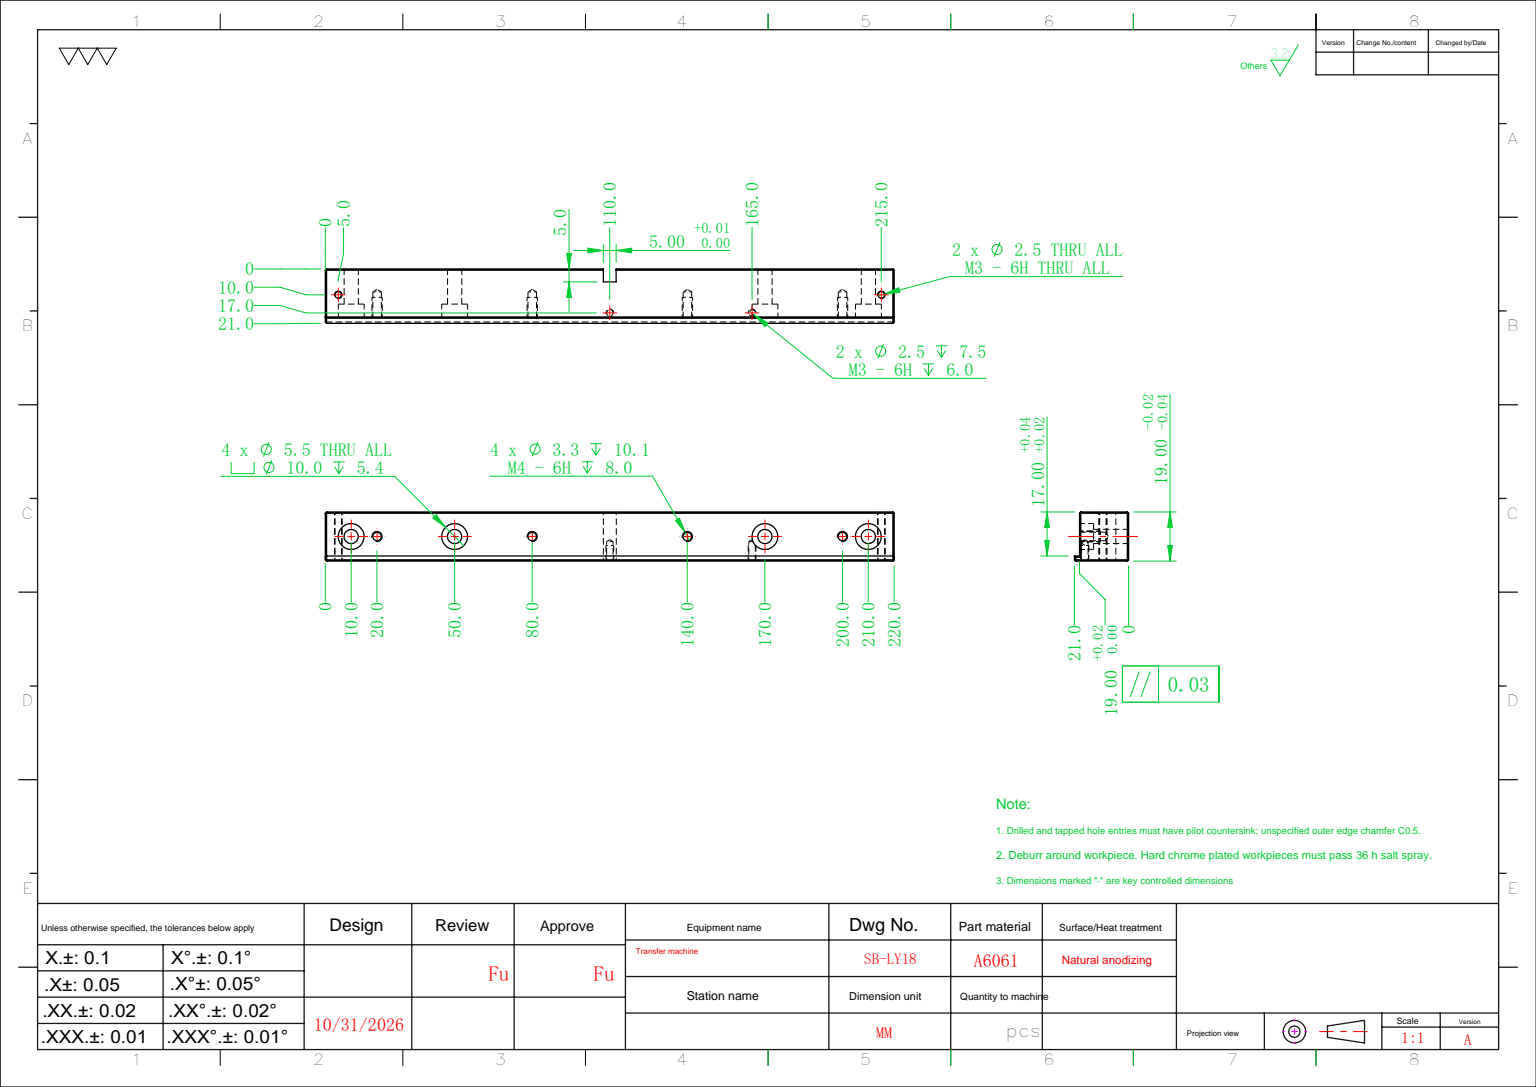
SolidWorks part; units mm, degrees
ref_plane "前视基准面" through (0, 0, 0) normal (0, 0, 1) x (1, 0, 0)
ref_plane "上视基准面" through (0, 0, 0) normal (0, 1, 0) x (1, 0, 0)
ref_plane "右视基准面" through (0, 0, 0) normal (1, 0, 0) x (0, 0, -1)
sketch "草图1" plane through (0, 0, 0) normal (0, 0, 1) x (1, 0, 0)
  line L1 (-110, -10.5) -> (110, -10.5)
  line L2 (-110, -10.5) -> (-110, 10.5)
  line L3 (-110, 10.5) -> (110, 10.5)
  line L4 (110, -10.5) -> (110, 10.5)
  line L5 (-110, -10.5) -> (110, 10.5) construction
  line L6 (-110, 10.5) -> (110, -10.5) construction
  point P0 (0, 0)
  dimension "D1" = 220
  dimension "D2" = 21
extrude "凸台-拉伸1" add sketch "草图1" along normal blind 19
sketch "草图2" plane through (0, -10.5, 0) normal (0, -1, 0) x (1, 0, 0)
  line L0 (110, 19) -> (110, 0) construction
  line L1 (110, 2) -> (-110, 2)
  line L2 (110, 2) -> (110, 17)
  line L3 (110, 17) -> (-110, 17)
  line L4 (-110, 2) -> (-110, 17)
  line L5 (-110, 19) -> (-110, 0) construction
  line L6 (-110, 9.5) -> (22.243, 9.5) construction
  dimension "D1" = 15
extrude "切除-拉伸1" cut sketch "草图2" against normal blind 2
hole_wizard "M4 螺纹孔1" positions "草图3" profile "草图4" tap size "M4" standard "ISO"
sketch "草图3" plane through (0, -8.5, 0) normal (0, -1, 0) x (-1, 0, 0)
  line L0 (-110, -9.5) -> (110, -9.5) construction
  line L1 (-110, -2) -> (-110, -17) construction
  line L2 (110, -17) -> (110, -2) construction
  point P0 (-90, -9.5)
  point P3 (-30, -9.5)
  point P6 (30, -9.5)
  point P24 (90, -9.5)
  dimension "D1" = 20
  dimension "D2" = 60
  dimension "D3" = 60
  dimension "D4" = 60
sketch "草图4" plane through (90, -8.5, 9.5) normal (1, 0, 0) x (0, 0, -1)
  line L0 (0, 0) -> (0, 11.0914)
  line L1 (0, 11.0914) -> (1.65, 10.1)
  line L2 (1.65, 10.1) -> (1.65, 0)
  line L5 (1.65, 0) -> (0, 0)
  line L10 (0, 11.0914) -> (-1.65, 10.1) construction
  line L11 (0, -6.35) -> (0, 107.95) construction
  dimension "螺纹孔钻头直径" = 3.3
  dimension "螺纹孔钻头深度" = 10.1
  dimension "导头角度" = 118
cosmetic thread "孔螺蚊线1" parameters "D1"=8, "D2"=4
cosmetic thread "孔螺蚊线2" parameters "D1"=8, "D2"=4
cosmetic thread "孔螺蚊线3" parameters "D1"=8, "D2"=4
cosmetic thread "孔螺蚊线6" parameters "D1"=8, "D2"=4
hole_wizard "M5 六角凹头螺钉的柱形沉头孔1" positions "草图5" profile "草图6" counterbore size "M5" standard "ISO" end condition through all
sketch "草图5" plane through (0, -8.5, 0) normal (0, -1, 0) x (-1, 0, 0)
  line L0 (110, -9.5) -> (-110, -9.5) construction
  line L1 (110, -17) -> (110, -2) construction
  line L2 (-110, -2) -> (-110, -17) construction
  line L4 (0, 0) -> (0, -30.2286) construction
  point P0 (-100, -9.5)
  point P2 (100, -9.5)
  point P16 (60, -9.5)
  point P18 (-60, -9.5)
  dimension "D1" = 200
  dimension "D2" = 40
sketch "草图6" plane through (100, -8.5, 9.5) normal (1, 0, 0) x (0, 0, -1)
  line L0 (0, 0) -> (0, 19)
  line L1 (0, 19) -> (2.75, 19)
  line L3 (2.75, 19) -> (2.75, 5.4)
  line L4 (2.75, 5.4) -> (5, 5.4)
  line L5 (5, 5.4) -> (5, 0)
  line L7 (5, 0) -> (0, 0)
  line L11 (0, -6.35) -> (0, 107.95) construction
  dimension "通孔孔直径" = 5.5
  dimension "通孔孔深度" = 19
  dimension "柱形沉头孔直径" = 10
  dimension "柱形沉头孔深度" = 5.4
sketch "草图7" plane through (0, 0, 19) normal (0, 0, 1) x (1, 0, 0)
  line L0 (110, 10.5) -> (-110, 10.5) construction
  line L1 (-2.5, 10.5) -> (2.5, 10.5)
  line L2 (-2.5, 10.5) -> (-2.5, 5.5)
  line L3 (-2.5, 5.5) -> (2.5, 5.5)
  line L4 (2.5, 10.5) -> (2.5, 5.5)
  line L5 (0, 0) -> (0, 16.0493) construction
  dimension "D1" = 5
  dimension "D2" = 5
extrude "切除-拉伸2" cut sketch "草图7" against normal through all
hole_wizard "M3 螺纹孔1" positions "草图8" profile "草图9" tap size "M3" standard "ISO"
sketch "草图8" plane through (0, 0, 0) normal (0, 0, -1) x (-1, 0, 0)
  line L0 (-110, -10.5) -> (-110, 10.5) construction
  line L1 (-110, 10.5) -> (-2.5, 10.5) construction
  point P0 (-55, -6.5)
  point P3 (0, -6.5)
  dimension "D1" = 55
  dimension "D2" = 17
  dimension "D3" = 55
sketch "草图9" plane through (55, -6.5, 0) normal (1, 0, 0) x (0, 1, 0)
  line L0 (0, 0) -> (0, 8.2511)
  line L1 (0, 8.2511) -> (1.25, 7.5)
  line L2 (1.25, 7.5) -> (1.25, 0)
  line L5 (1.25, 0) -> (0, 0)
  line L10 (0, 8.2511) -> (-1.25, 7.5) construction
  line L11 (0, -6.35) -> (0, 107.95) construction
  dimension "螺纹孔钻头直径" = 2.5
  dimension "螺纹孔钻头深度" = 7.5
  dimension "导头角度" = 118
cosmetic thread "孔螺蚊线4" parameters "D1"=6, "D2"=3
cosmetic thread "孔螺蚊线5" parameters "D1"=6, "D2"=3
sketch "草图12" plane through (110, 0, 0) normal (1, 0, 0) x (0, 0, -1)
  line L0 (-19, -10.5) -> (-19, 10.5) construction
  line L1 (-19, -8.5) -> (-17, -8.5)
  line L2 (-19, -8.5) -> (-19, -10.5)
  line L3 (-19, -10.5) -> (-17, -10.5)
  line L4 (-17, -8.5) -> (-17, -10.5)
extrude "切除-拉伸3" cut sketch "草图12" against normal through all
chamfer "倒角1" distance 0.5 angle 45 18 edges at (110, 1, 19) (56.25, 10.5, 19) (110, 10.5, 9.5) (110, -8.5, 10.5) (110, -9.5, 2) (110, -10.5, 1) (-110, 0, 0) (-56.25, 10.5, 0) (-110, 10.5, 9.5) (-56.25, 10.5, 19) (-110, 1, 19) (-110, -8.5, 10.5) (-110, -9.5, 2) (-110, -10.5, 1) (0, -10.5, 0) (110, 0, 0) (56.25, 10.5, 0) (0, -8.5, 19)
hole_wizard "M3 螺纹孔2" positions "草图10" profile "草图11" tap size "M3" standard "ISO" end condition through all
sketch "草图10" plane through (0, 0, 0) normal (0, 0, -1) x (-1, 0, 0)
  line L0 (0, 0) -> (0, 23.9769) construction
  line L2 (2.5, 10.5) -> (109.5, 10.5) construction
  point P0 (105, 0.5)
  point P2 (-105, 0.5)
  dimension "D1" = 210
  dimension "D2" = 10
sketch "草图11" plane through (-105, 0.5, 0) normal (1, 0, 0) x (0, 1, 0)
  line L0 (0, 0) -> (0, 19)
  line L1 (0, 19) -> (1.25, 19)
  line L2 (1.25, 19) -> (1.25, 0)
  line L5 (1.25, 0) -> (0, 0)
  line L11 (0, -6.35) -> (0, 107.95) construction
  dimension "通孔螺纹孔钻头直径" = 2.5
  dimension "通孔螺纹孔钻头深度" = 19
cosmetic thread "孔螺蚊线7" parameters "D2"=3
cosmetic thread "孔螺蚊线8" parameters "D2"=3
